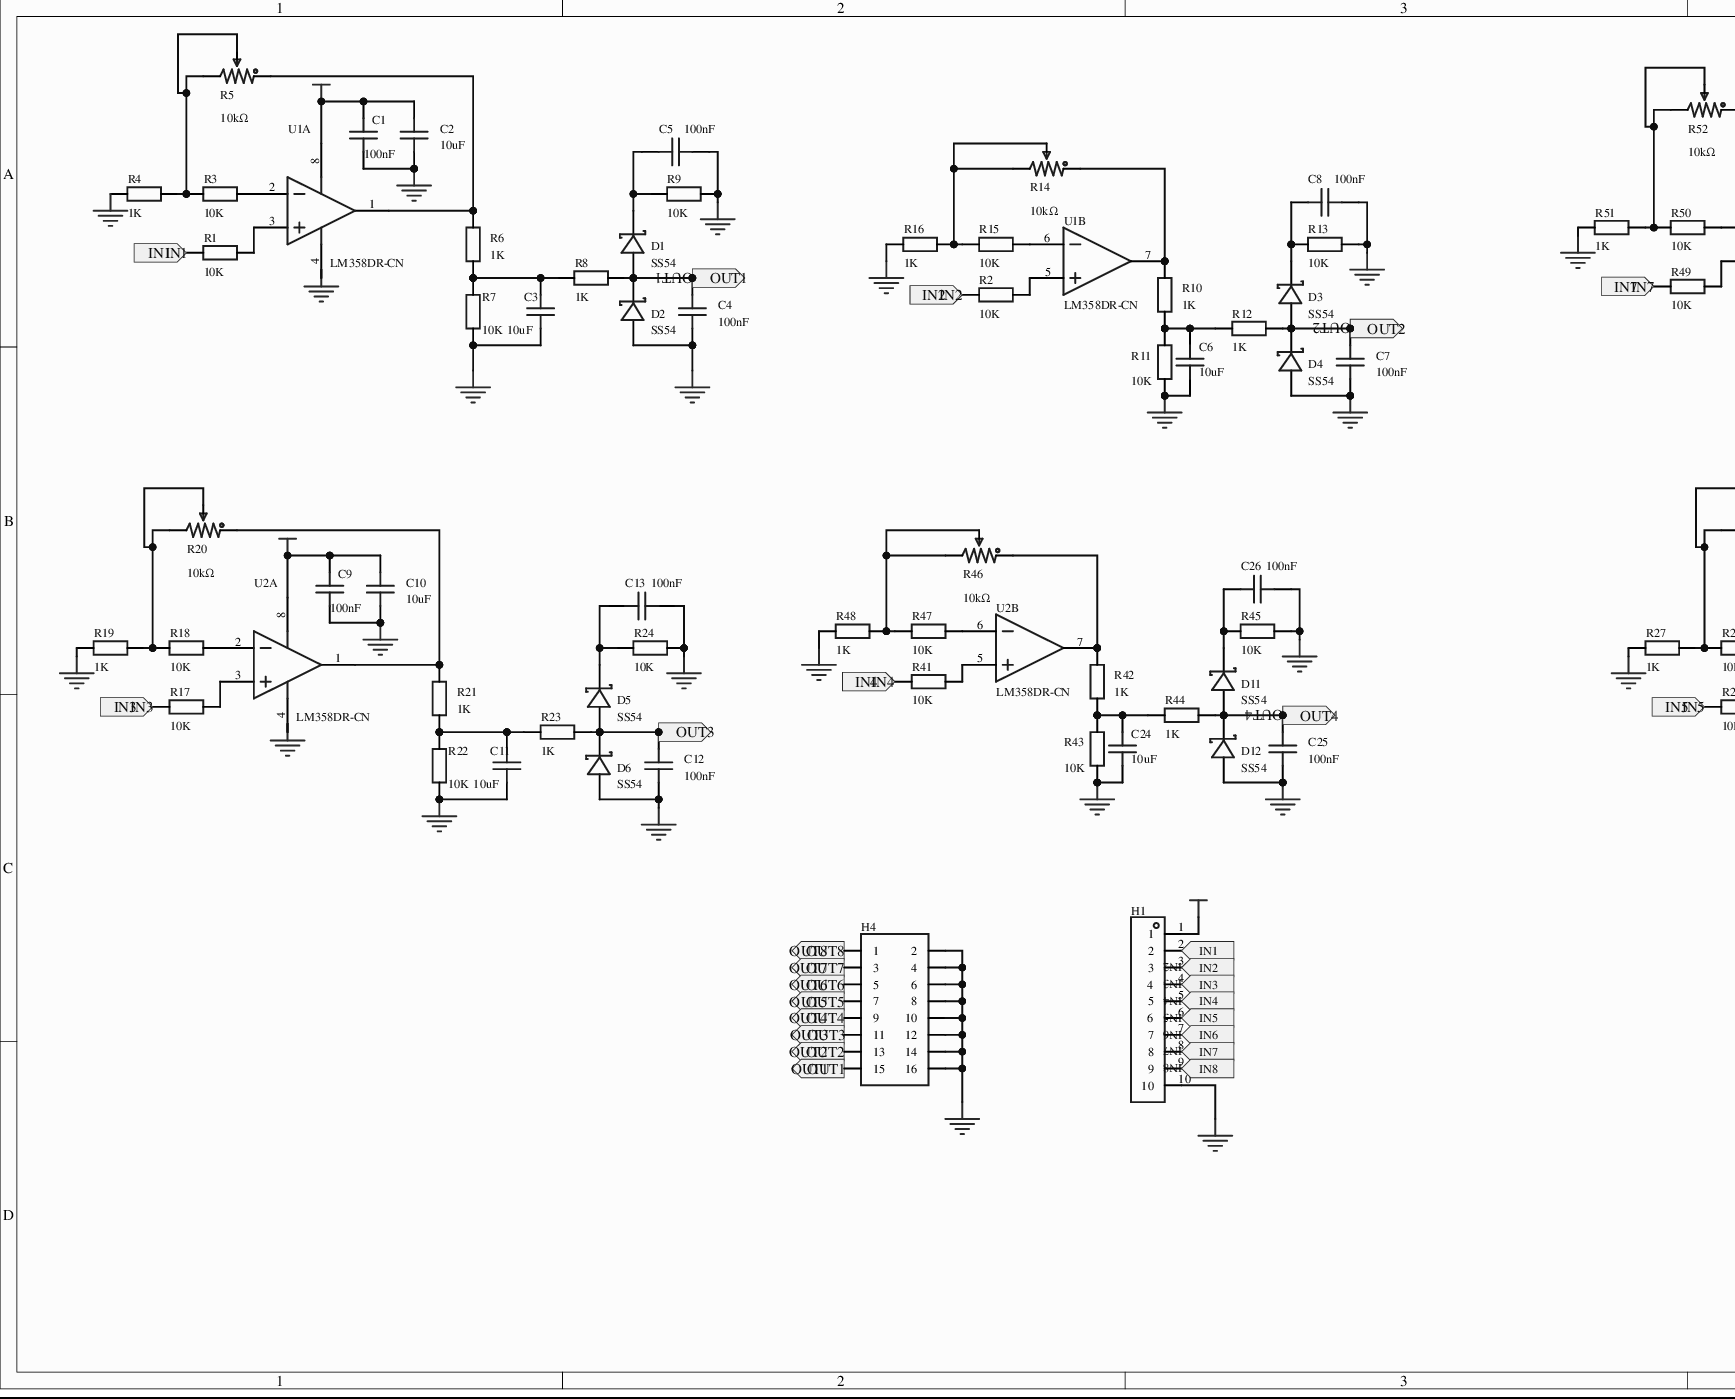
[diagram p0: MISC49941-3.schdoc, left]
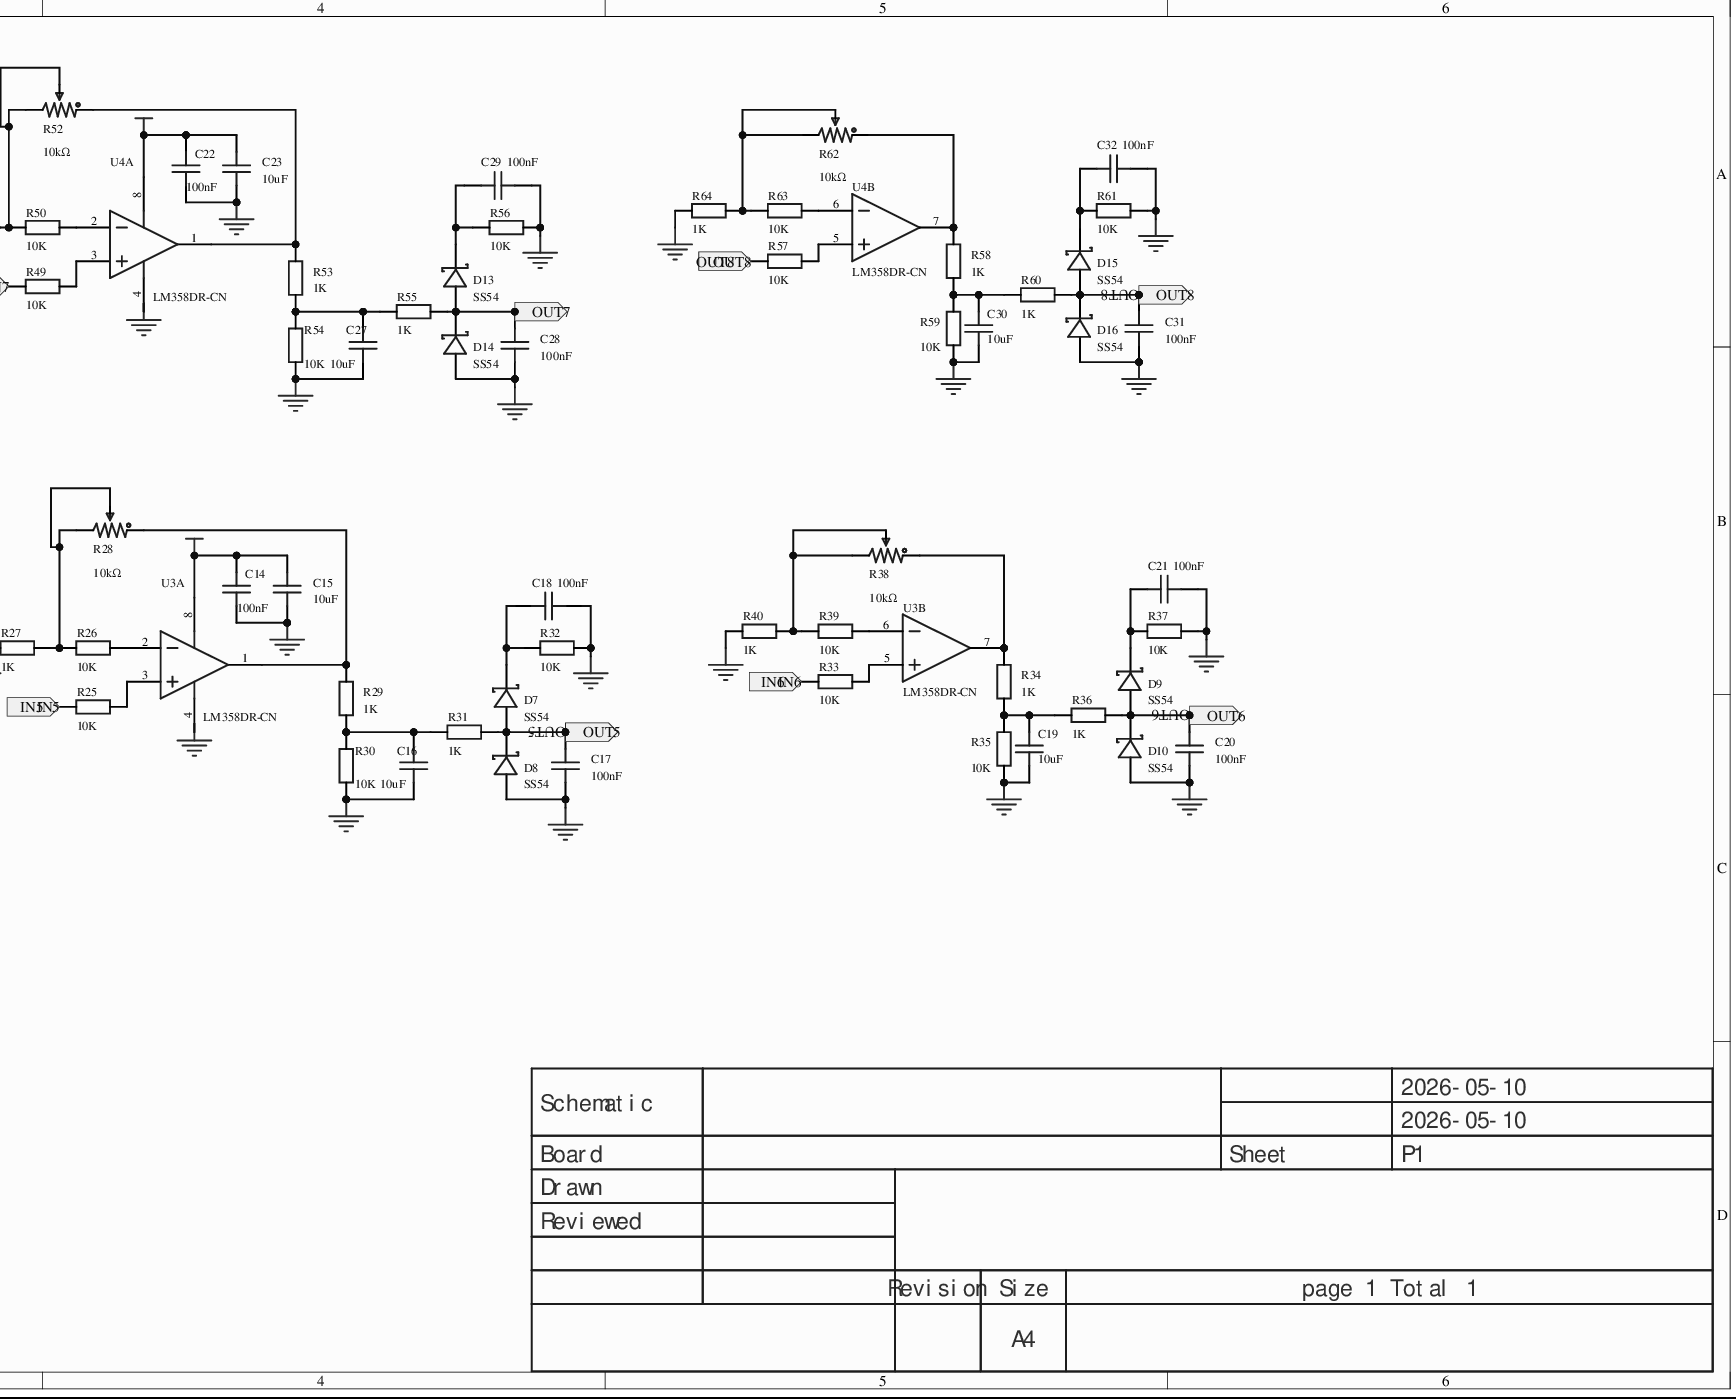
[diagram p1: MISC49941-3.schdoc, right]
# Altium project MISC49941-2.PrjPcb
1 sheet, 118 parts. Net scope: flat (ports and power ports of the same name join across sheets).
Board file: MISC49941.pcbdoc

## Sheet MISC49941-3.schdoc
size 508 x 209 mm; Version: V1.0; @Project Name: MISC49941; @Update Date: 2026-05-10; @Create Date: 2026-05-10; @Board Name: MISC49941; @Create Time: 23:07:01; @Page Count: 1; @Page No: 1; @Schematic Name: MISC49941; @Update Time: 23:07:01; Size: A4

### Parts
C1  100nF  [C0603]
C2  10uF  [C0603]
C3  10uF  [C0603]
C4  100nF  [C0603]
C5  100nF  [C0603]
C6  10uF  [C0603]
C7  100nF  [C0603]
C8  100nF  [C0603]
C9  100nF  [C0603]
C10  10uF  [C0603]
C11  10uF  [C0603]
C12  100nF  [C0603]
C13  100nF  [C0603]
C14  100nF  [C0603]
C15  10uF  [C0603]
C16  10uF  [C0603]
C17  100nF  [C0603]
C18  100nF  [C0603]
C19  10uF  [C0603]
C20  100nF  [C0603]
C21  100nF  [C0603]
C22  100nF  [C0603]
C23  10uF  [C0603]
C24  10uF  [C0603]
C25  100nF  [C0603]
C26  100nF  [C0603]
C27  10uF  [C0603]
C28  100nF  [C0603]
C29  100nF  [C0603]
C30  10uF  [C0603]
C31  100nF  [C0603]
C32  100nF  [C0603]
D1  SS54  [SMA_L4.4-W2.8-LS5.4-R-RD]
D2  SS54  [SMA_L4.4-W2.8-LS5.4-R-RD]
D3  SS54  [SMA_L4.4-W2.8-LS5.4-R-RD]
D4  SS54  [SMA_L4.4-W2.8-LS5.4-R-RD]
D5  SS54  [SMA_L4.4-W2.8-LS5.4-R-RD]
D6  SS54  [SMA_L4.4-W2.8-LS5.4-R-RD]
D7  SS54  [SMA_L4.4-W2.8-LS5.4-R-RD]
D8  SS54  [SMA_L4.4-W2.8-LS5.4-R-RD]
D9  SS54  [SMA_L4.4-W2.8-LS5.4-R-RD]
D10  SS54  [SMA_L4.4-W2.8-LS5.4-R-RD]
D11  SS54  [SMA_L4.4-W2.8-LS5.4-R-RD]
D12  SS54  [SMA_L4.4-W2.8-LS5.4-R-RD]
D13  SS54  [SMA_L4.4-W2.8-LS5.4-R-RD]
D14  SS54  [SMA_L4.4-W2.8-LS5.4-R-RD]
D15  SS54  [SMA_L4.4-W2.8-LS5.4-R-RD]
D16  SS54  [SMA_L4.4-W2.8-LS5.4-R-RD]
H1  (no value)  [HDR-TH_10P-P2.54-V-F]
H4  (no value)  [HDR-TH_16P-P2.54-V-F-R2-C8-S2.54-1]
R1  10K  [R0603]
R2  10K  [R0603]
R3  10K  [R0603]
R4  1K  [R0603]
R5  10kΩ  [RES-ADJ-TH_3P-L10.0-W10.0-P2.50-L]
R6  1K  [R0603]
R7  10K  [R0603]
R8  1K  [R0603]
R9  10K  [R0603]
R10  1K  [R0603]
R11  10K  [R0603]
R12  1K  [R0603]
R13  10K  [R0603]
R14  10kΩ  [RES-ADJ-TH_3P-L10.0-W10.0-P2.50-L]
R15  10K  [R0603]
R16  1K  [R0603]
R17  10K  [R0603]
R18  10K  [R0603]
R19  1K  [R0603]
R20  10kΩ  [RES-ADJ-TH_3P-L10.0-W10.0-P2.50-L]
R21  1K  [R0603]
R22  10K  [R0603]
R23  1K  [R0603]
R24  10K  [R0603]
R25  10K  [R0603]
R26  10K  [R0603]
R27  1K  [R0603]
R28  10kΩ  [RES-ADJ-TH_3P-L10.0-W10.0-P2.50-L]
R29  1K  [R0603]
R30  10K  [R0603]
R31  1K  [R0603]
R32  10K  [R0603]
R33  10K  [R0603]
R34  1K  [R0603]
R35  10K  [R0603]
R36  1K  [R0603]
R37  10K  [R0603]
R38  10kΩ  [RES-ADJ-TH_3P-L10.0-W10.0-P2.50-L]
R39  10K  [R0603]
R40  1K  [R0603]
R41  10K  [R0603]
R42  1K  [R0603]
R43  10K  [R0603]
R44  1K  [R0603]
R45  10K  [R0603]
R46  10kΩ  [RES-ADJ-TH_3P-L10.0-W10.0-P2.50-L]
R47  10K  [R0603]
R48  1K  [R0603]
R49  10K  [R0603]
R50  10K  [R0603]
R51  1K  [R0603]
R52  10kΩ  [RES-ADJ-TH_3P-L10.0-W10.0-P2.50-L]
R53  1K  [R0603]
R54  10K  [R0603]
R55  1K  [R0603]
R56  10K  [R0603]
R57  10K  [R0603]
R58  1K  [R0603]
R59  10K  [R0603]
R60  1K  [R0603]
R61  10K  [R0603]
R62  10kΩ  [RES-ADJ-TH_3P-L10.0-W10.0-P2.50-L]
R63  10K  [R0603]
R64  1K  [R0603]
U1  LM358DR-CN  [SOIC-8_L4.9-W4.0-P1.27-LS6.0-BL]  (parts A,B of 2)
U2  LM358DR-CN  [SOIC-8_L4.9-W4.0-P1.27-LS6.0-BL]  (parts A,B of 2)
U3  LM358DR-CN  [SOIC-8_L4.9-W4.0-P1.27-LS6.0-BL]  (parts A,B of 2)
U4  LM358DR-CN  [SOIC-8_L4.9-W4.0-P1.27-LS6.0-BL]  (parts A,B of 2)

### Ports
IN1 (in), IN2 (in), IN3 (in), IN4 (in), IN5 (in), IN6 (in), IN7 (in), IN8 (in), OUT1 (out), OUT2 (out), OUT3 (out), OUT4 (out), OUT5 (out), OUT6 (out), OUT7 (out), OUT8 (in), OUT8 (out)

### Nets
+5V: C1.2 C2.2 C9.2 C10.2 C14.2 C15.2 C22.2 C23.2 H1.1 U1.8(V+) U2.8(V+) U3.8(V+) U4.8(V+)
GND: C1.1 C2.1 C3.1 C4.1 C5.1 C6.1 C7.1 C8.1 C9.1 C10.1 C11.1 C12.1 C13.1 C14.1 C15.1 C16.1 C17.1 C18.1 C19.1 C20.1 C21.1 C22.1 C23.1 C24.1 C25.1 C26.1 C27.1 C28.1 C29.1 C30.1 C31.1 C32.1 D2.1(A) D4.1(A) D6.1(A) D8.1(A) D10.1(A) D12.1(A) D14.1(A) D16.1(A) H1.10 H4.2 H4.4 H4.6 H4.8 H4.10 H4.12 H4.14 H4.16 R4.1 R7.1 R9.2 R11.1 R13.2 R16.1 R19.1 R22.1 R24.2 R27.1 R30.1 R32.2 R35.1 R37.2 R40.1 R43.1 R45.2 R48.1 R51.1 R54.1 R56.2 R59.1 R61.2 R64.1 U1.4(V-) U2.4(V-) U3.4(V-) U4.4(V-)
IN1: H1.2 R1.1 ; port IN1
IN2: H1.3 R2.1 ; port IN2
IN3: H1.4 R17.1 ; port IN3
IN4: H1.5 R41.1 ; port IN4
IN5: H1.6 R25.1 ; port IN5
IN6: H1.7 R33.1 ; port IN6
IN7: H1.8 R49.1 ; port IN7
IN8: H1.9 ; port IN8
OUT1: C4.2 D1.1(A) D2.2(K) H4.15 R8.2 ; port OUT1
OUT2: C7.2 D3.1(A) D4.2(K) H4.13 R12.2 ; port OUT2
OUT3: C12.2 D5.1(A) D6.2(K) H4.11 R23.2 ; port OUT3
OUT4: C25.2 D11.1(A) D12.2(K) H4.9 R44.2 ; port OUT4
OUT5: C17.2 D7.1(A) D8.2(K) H4.7 R31.2 ; port OUT5
OUT6: C20.2 D9.1(A) D10.2(K) H4.5 R36.2 ; port OUT6
OUT7: C28.2 D13.1(A) D14.2(K) H4.3 R55.2 ; port OUT7
OUT8: C31.2 D15.1(A) D16.2(K) H4.1 R57.1 R60.2 ; port OUT8
NetC3_2: C3.2 R6.1 R7.2 R8.1
NetC5_2: C5.2 D1.2(K) R9.1
NetC6_2: C6.2 R10.1 R11.2 R12.1
NetC8_2: C8.2 D3.2(K) R13.1
NetC11_2: C11.2 R21.1 R22.2 R23.1
NetC13_2: C13.2 D5.2(K) R24.1
NetC16_2: C16.2 R29.1 R30.2 R31.1
NetC18_2: C18.2 D7.2(K) R32.1
NetC19_2: C19.2 R34.1 R35.2 R36.1
NetC21_2: C21.2 D9.2(K) R37.1
NetC24_2: C24.2 R42.1 R43.2 R44.1
NetC26_2: C26.2 D11.2(K) R45.1
NetC27_2: C27.2 R53.1 R54.2 R55.1
NetC29_2: C29.2 D13.2(K) R56.1
NetC30_2: C30.2 R58.1 R59.2 R60.1
NetC32_2: C32.2 D15.2(K) R61.1
NetR1_2: R1.2 U1.3(IN1+)
NetR2_2: R2.2 U1.5(IN2+)
NetR3_1: R3.1 R4.2 R5.2 R5.3
NetR3_2: R3.2 U1.2(IN1-)
NetR5_1: R5.1 R6.2 U1.1(OUT1)
NetR10_2: R10.2 R14.1 U1.7(OUT2)
NetR14_2: R14.2 R14.3 R15.1 R16.2
NetR15_2: R15.2 U1.6(IN2-)
NetR17_2: R17.2 U2.3(IN1+)
NetR18_1: R18.1 R19.2 R20.2 R20.3
NetR18_2: R18.2 U2.2(IN1-)
NetR20_1: R20.1 R21.2 U2.1(OUT1)
NetR25_2: R25.2 U3.3(IN1+)
NetR26_1: R26.1 R27.2 R28.2 R28.3
NetR26_2: R26.2 U3.2(IN1-)
NetR28_1: R28.1 R29.2 U3.1(OUT1)
NetR33_2: R33.2 U3.5(IN2+)
NetR34_2: R34.2 R38.1 U3.7(OUT2)
NetR38_2: R38.2 R38.3 R39.1 R40.2
NetR39_2: R39.2 U3.6(IN2-)
NetR41_2: R41.2 U2.5(IN2+)
NetR42_2: R42.2 R46.1 U2.7(OUT2)
NetR46_2: R46.2 R46.3 R47.1 R48.2
NetR47_2: R47.2 U2.6(IN2-)
NetR49_2: R49.2 U4.3(IN1+)
NetR50_1: R50.1 R51.2 R52.2 R52.3
NetR50_2: R50.2 U4.2(IN1-)
NetR52_1: R52.1 R53.2 U4.1(OUT1)
NetR57_2: R57.2 U4.5(IN2+)
NetR58_2: R58.2 R62.1 U4.7(OUT2)
NetR62_2: R62.2 R62.3 R63.1 R64.2
NetR63_2: R63.2 U4.6(IN2-)

### Notes on the sheet
- 2026-05-10
- Schematic
- Board
- Sheet
- P1
- Drawn
- Reviewed
- Revision
- Size
- A4
- page 1 Total 1

### Library data of the parts
C1-C32 = CAP_0603: Symbol: Capacitance; 3D Model: ac125912035d415993ca9572d50418b1; 3D Model Transform: 62.992,31.496,0,0,0,0,0,0,0; ConvertToPcb: yes; ModelName: C0603_L1.6-W0.8-H0.8; Device: CAP_0603; Supplier Footprint: 0603; AddInBom: yes; FootprintName: C0603
  C1 C4 C5 C7-C9 C12-C14 C17 C18 C20-C22 C25 C26 C28 C29 C31 C32: Value: 100nF
  C2 C3 C6 C10 C11 C15 C16 C19 C23 C24 C27 C30: Value: 10uF
D1-D16 = SS54_C22452: Diode configuration: Single; Forward voltage (Vf): 550mV@5A; DC reverse voltage (Vr): 40V; Rectifier current: 5A;; Manufacturer: MDD(辰达半导体); 3D Model: 228de99b63224bd3982b21290755dd84; 3D Model Transform: 204.724,110.236,0,0,0,0,0,0,0; Reverse Leakage Current (Ir): 1mA@40V; AddInBom: yes; Symbol: SS54_C22452; Device: SS54_C22452; LCSC Part Name: 电压:40V 电流:5A; Supplier Part: C22452; Manufacturer Part: SS54; Supplier Footprint: SMA(DO-214AC); JLCPCB Part Class: Basic library; Datasheet: https://atta.szlcsc.com/upload/public/pdf/source/20240710/73DFBB65C1883B895E62D589679033DF.pdf; Supplier: LCSC; Diode Configuration: Single; Forward Voltage (Vf@If): 550mV@5A; Reverse Voltage (Vr): 40V; Rectified Current: 5A; ConvertToPcb: yes; FootprintName: SMA_L4.4-W2.8-LS5.4-R-RD; ModelName: SMA_L4.4-W2.8-LS5.4-R-RD
H1 = HDR-F_2.54_1x10P: Symbol: X5511FV-10-C70D30-1000; 3D Model: 08a5ee31ec6747838a696d2ac093ffa4; 3D Model Transform: 1009.87987,100,0,0,0,0,0,0,-125.984; AddInBom: yes; ModelName: HDR-TH_10P-P2.54-F-LI-1X10P; Device: HDR-F_2.54_1x10P; Supplier Part: C2684744; Supplier Footprint: 插件; ConvertToPcb: yes; FootprintName: HDR-TH_10P-P2.54-V-F
H4 = HDR-F_2.54_2x8: Symbol: HDR-F-2.54_2x8; 3D Model: f6b5f7d40ec74b809fbaeebc5002f6e00819f05c4eef4c71ace90d822a990e87; 3D Model Transform: 799.99844,200,0,0,0,0,0,0,-118.11; ConvertToPcb: yes; ModelName: HDR2.54-F-LI-2X8P; Device: HDR-F_2.54_2x8; Supplier Part: C30734; Supplier Footprint: 插件; AddInBom: yes; FootprintName: HDR-TH_16P-P2.54-V-F-R2-C8-S2.54-1
R1-R4 R6-R13 R15-R19 R21-R27 R29-R37 R39-R45 R47-R51 R53-R61 R63 R64 = Res_0603: Symbol: Resistor; 3D Model: fc143cca1e79419f9cd78b61e9279f08; 3D Model Transform: 31.8897,63.7794,0,90,0,0,0,0,0; ConvertToPcb: yes; Device: Res_0603; Supplier Footprint: 0603; AddInBom: yes; FootprintName: R0603; ModelName: R0603
  R1-R3 R7 R9 R11 R13 R15 R17 R18 R22 R24-R26 R30 R32 R33 R35 R37 R39 R41 R43 R45 R47 R49 R50 R54 R56 R57 R59 R61 R63: Value: 10K
  R4 R6 R8 R10 R12 R16 R19 R21 R23 R27 R29 R31 R34 R36 R40 R42 R44 R48 R51 R53 R55 R58 R60 R64: Value: 1K
R5 R14 R20 R28 R38 R46 R52 R62 = 3296W-1-103: Resistance: 10kΩ; Tolerance: ±10%;; Manufacturer: BOCHEN(博晨); 3D Model: b182808559bb43bda9e7de64b64134cb; 3D Model Transform: 374.015,188.976,0,180,0,0,0,0,-137.795; AddInBom: yes; ModelName: 3296W; Symbol: 3296W-1-103; Device: 3296W-1-103; LCSC Part Name: 10kΩ ±10%; Supplier Part: C118954; Manufacturer Part: 3296W-1-103; Supplier Footprint: 插件; JLCPCB Part Class: Extended library; Datasheet: https://atta.szlcsc.com/upload/public/pdf/source/20171114/C118954_15106326646611117443.pdf; Supplier: LCSC; Value: 10kΩ; Tolerance: ±10%; ConvertToPcb: yes; FootprintName: RES-ADJ-TH_3P-L10.0-W10.0-P2.50-L
U1-U4 = LM358DR-CN: Manufacturer: ChipNobo(无边界); Relevance: []; 3D Model: f04b1702bced497a80c713fe4e712e0c; 3D Model Transform: 192.913,238.9759,0,0,0,0,0,0,0; AddInBom: yes; Symbol: LM358DR-CN; Device: LM358DR-CN; LCSC Part Name: LM358DR-CN; Supplier Part: C42436860; Manufacturer Part: LM358DR-CN; Supplier Footprint: SOP-8; Datasheet: https://atta.szlcsc.com/upload/public/pdf/source/20250107/27260A6478C0357093F3C3E006771478.pdf; Supplier: LCSC; ConvertToPcb: yes; FootprintName: SOIC-8_L4.9-W4.0-P1.27-LS6.0-BL; ModelName: SOIC-8_L4.9-W4.0-P1.27-LS6.0-BL